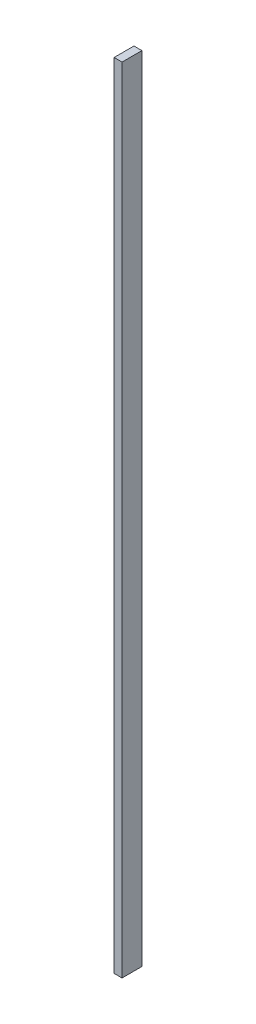
SolidWorks part; units mm, degrees
ref_plane "Front Plane" through (0, 0, 0) normal (0, 0, 1) x (1, 0, 0)
ref_plane "Top Plane" through (0, 0, 0) normal (0, 1, 0) x (1, 0, 0)
ref_plane "Right Plane" through (0, 0, 0) normal (1, 0, 0) x (0, 0, -1)
sketch "Sketch1" plane through (0, 0, 0) normal (1, 0, 0) x (0, 0, -1)
  line L1 (0, 0) -> (50, 0)
  line L2 (0, 0) -> (0, 1996)
  line L3 (0, 1996) -> (50, 1996)
  line L4 (50, 0) -> (50, 1996)
  dimension "D1" = 50
  dimension "D2" = 1996
extrude "Boss-Extrude1" add sketch "Sketch1" along normal blind 20
